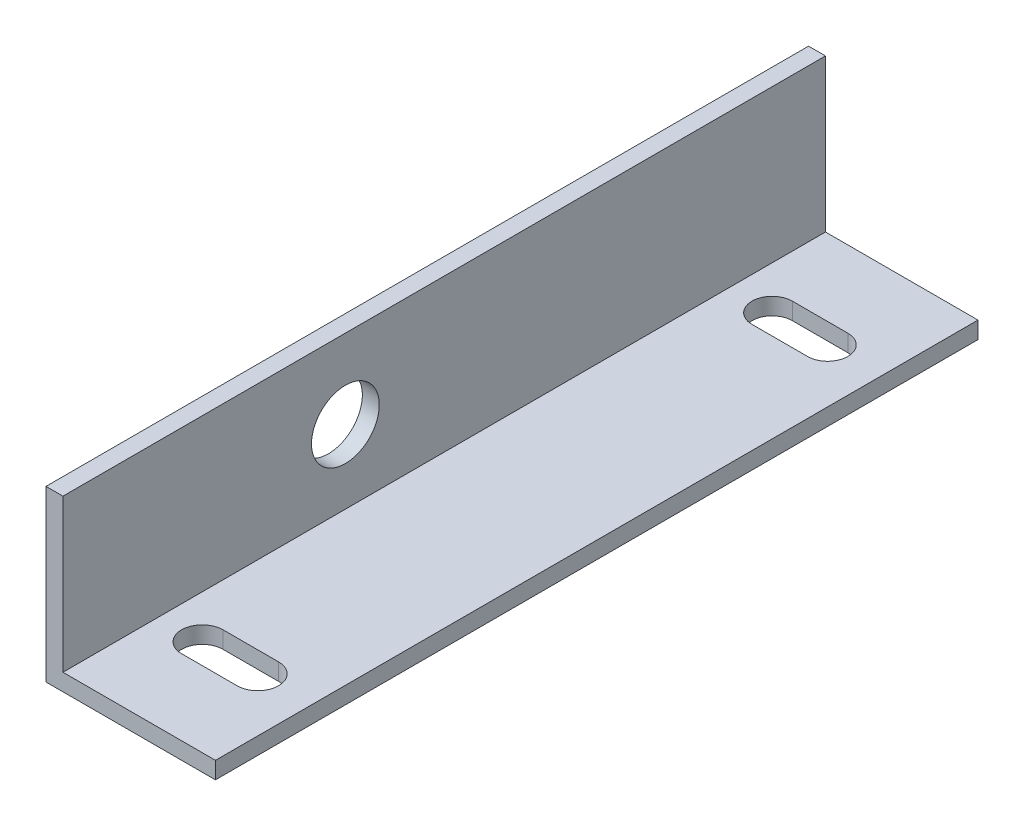
from build123d import *

# Parameters (mm, degrees)
BOSS_EXTRUDE1_DEPTH = 135
CUT_EXTRUDE1_DEPTH  = 160
SKETCH3_R           = 6
CUT_EXTRUDE2_DEPTH  = 10


with BuildPart() as part:
    # Sketch1 → Boss-Extrude1 (new body)
    with BuildSketch(Plane.XY):
        Polygon((0, 0), (0, 30), (3, 30), (3, 3), (30, 3), (30, 0), align=None)
    extrude(amount=BOSS_EXTRUDE1_DEPTH)

    # Sketch2 → Cut-Extrude1 (cut)
    with BuildSketch(Plane(origin=(0, 3, 0), x_dir=(1, 0, 0), z_dir=(0, 1, 0))):
        with BuildLine():
            Line((10.658971341, -13.531915857), (20.494612748, -13.531915857))
            ThreePointArc((20.494612748, -13.531915857), (24.063483391, -17.1007865), (20.494612748, -20.669657144))
            Line((20.494612748, -20.669657144), (10.658971341, -20.669657144))
            ThreePointArc((10.658971341, -20.669657144), (7.090100697, -17.1007865), (10.658971341, -13.531915857))
        make_face()
        with BuildLine():
            Line((10.658971341, -114.317792599), (20.494612748, -114.317792599))
            ThreePointArc((20.494612748, -114.317792599), (24.161447744, -117.984627595), (20.494612748, -121.65146259))
            Line((20.494612748, -121.65146259), (10.658971341, -121.65146259))
            ThreePointArc((10.658971341, -121.65146259), (6.992136345, -117.984627595), (10.658971341, -114.317792599))
        make_face()
    extrude(amount=-CUT_EXTRUDE1_DEPTH, mode=Mode.SUBTRACT)

    # Sketch3 → Cut-Extrude2 (cut)
    with BuildSketch(Plane.ZY):
        with Locations((85, 16)):
            Circle(SKETCH3_R)
    extrude(amount=-CUT_EXTRUDE2_DEPTH, mode=Mode.SUBTRACT)


solid = part.part
